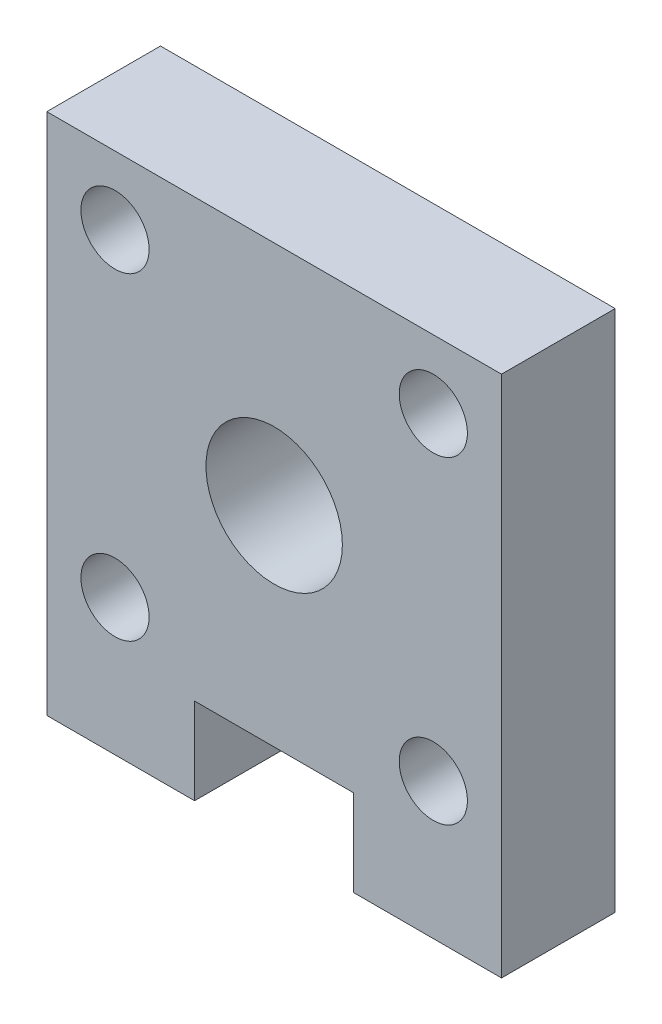
SolidWorks part; units mm, degrees
ref_plane "Front Plane" through (0, 0, 0) normal (0, 0, 1) x (1, 0, 0)
ref_plane "Top Plane" through (0, 0, 0) normal (0, 1, 0) x (1, 0, 0)
ref_plane "Right Plane" through (0, 0, 0) normal (1, 0, 0) x (0, 0, -1)
sketch "Sketch1" plane through (0, 0, 0) normal (0, 0, 1) x (1, 0, 0)
  line L2 (-10, -10) -> (-10, 10)
  line L3 (-10, 10) -> (-5, 10)
  line L4 (10, -10) -> (10, 10)
  line L5 (3.5, -13) -> (3.5, -9.2)
  line L9 (10, -10) -> (10, -13)
  line L10 (10, -13) -> (3.5, -13)
  line L11 (-10, -10) -> (-10, -13)
  line L12 (3.5, -9.2) -> (-3.5, -9.2)
  line L13 (-3.5, -9.2) -> (-3.5, -13)
  line L14 (-3.5, -13) -> (-10, -13)
  line L22 (5, 10) -> (10, 10)
  line L23 (5, 10) -> (-5, 10)
  circle A1 centre (0, 0) radius 3
  circle A2 centre (-7, 7) radius 1.5
  circle A3 centre (7, 7) radius 1.5
  circle A4 centre (7, -7) radius 1.5
  circle A5 centre (-7, -7) radius 1.5
  dimension "D1" = 6
  dimension "D2" = 20
  dimension "D4" = 3
  dimension "D5" = 3
  dimension "D6" = 3
  dimension "D7" = 3
  dimension "D9" = 3
  dimension "D11" = 3
  dimension "D3" = 20
  dimension "D8" = 3
  dimension "D10" = 3
  dimension "D12" = 3
  dimension "D13" = 3.8
  dimension "D14" = 7
  dimension "D15" = 3.5
extrude "Boss-Extrude1" add sketch "Sketch1" along normal blind 5
